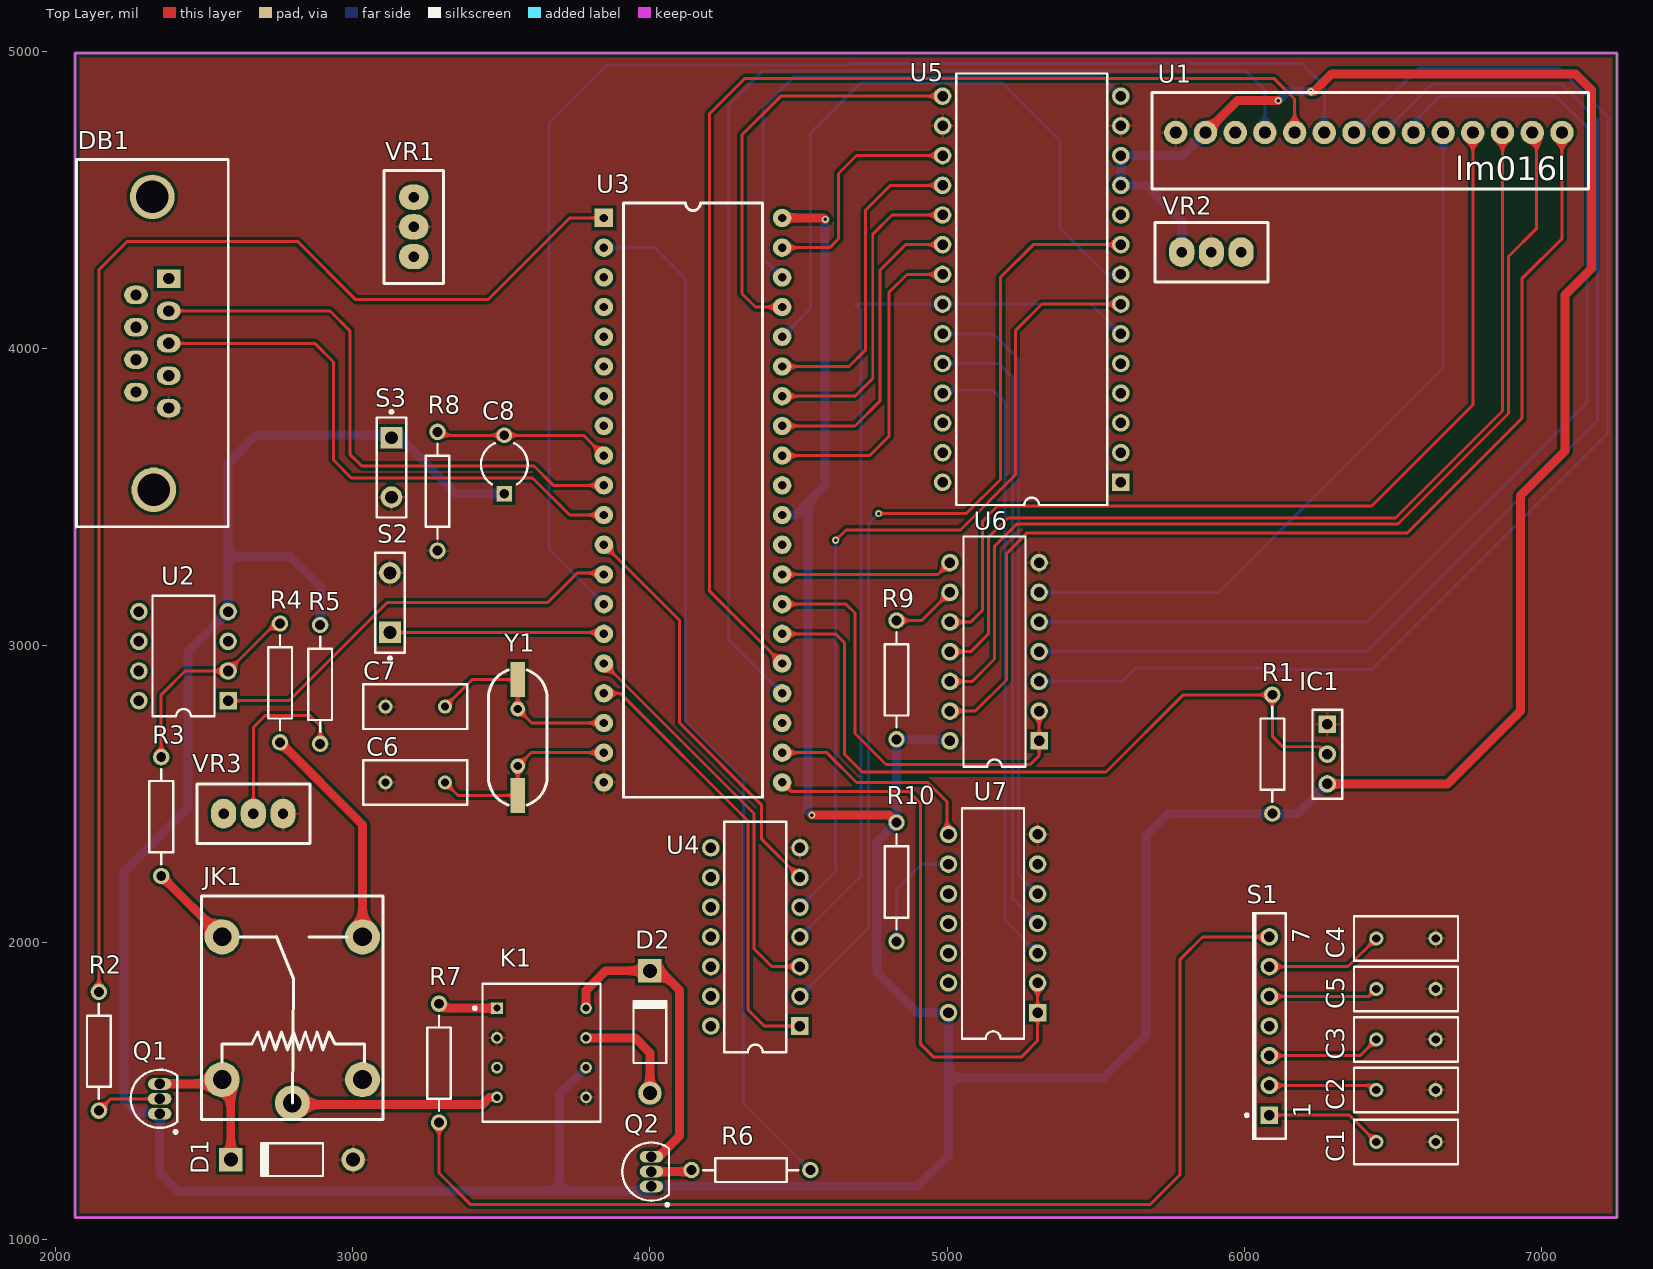
[diagram p0: Top Layer view]
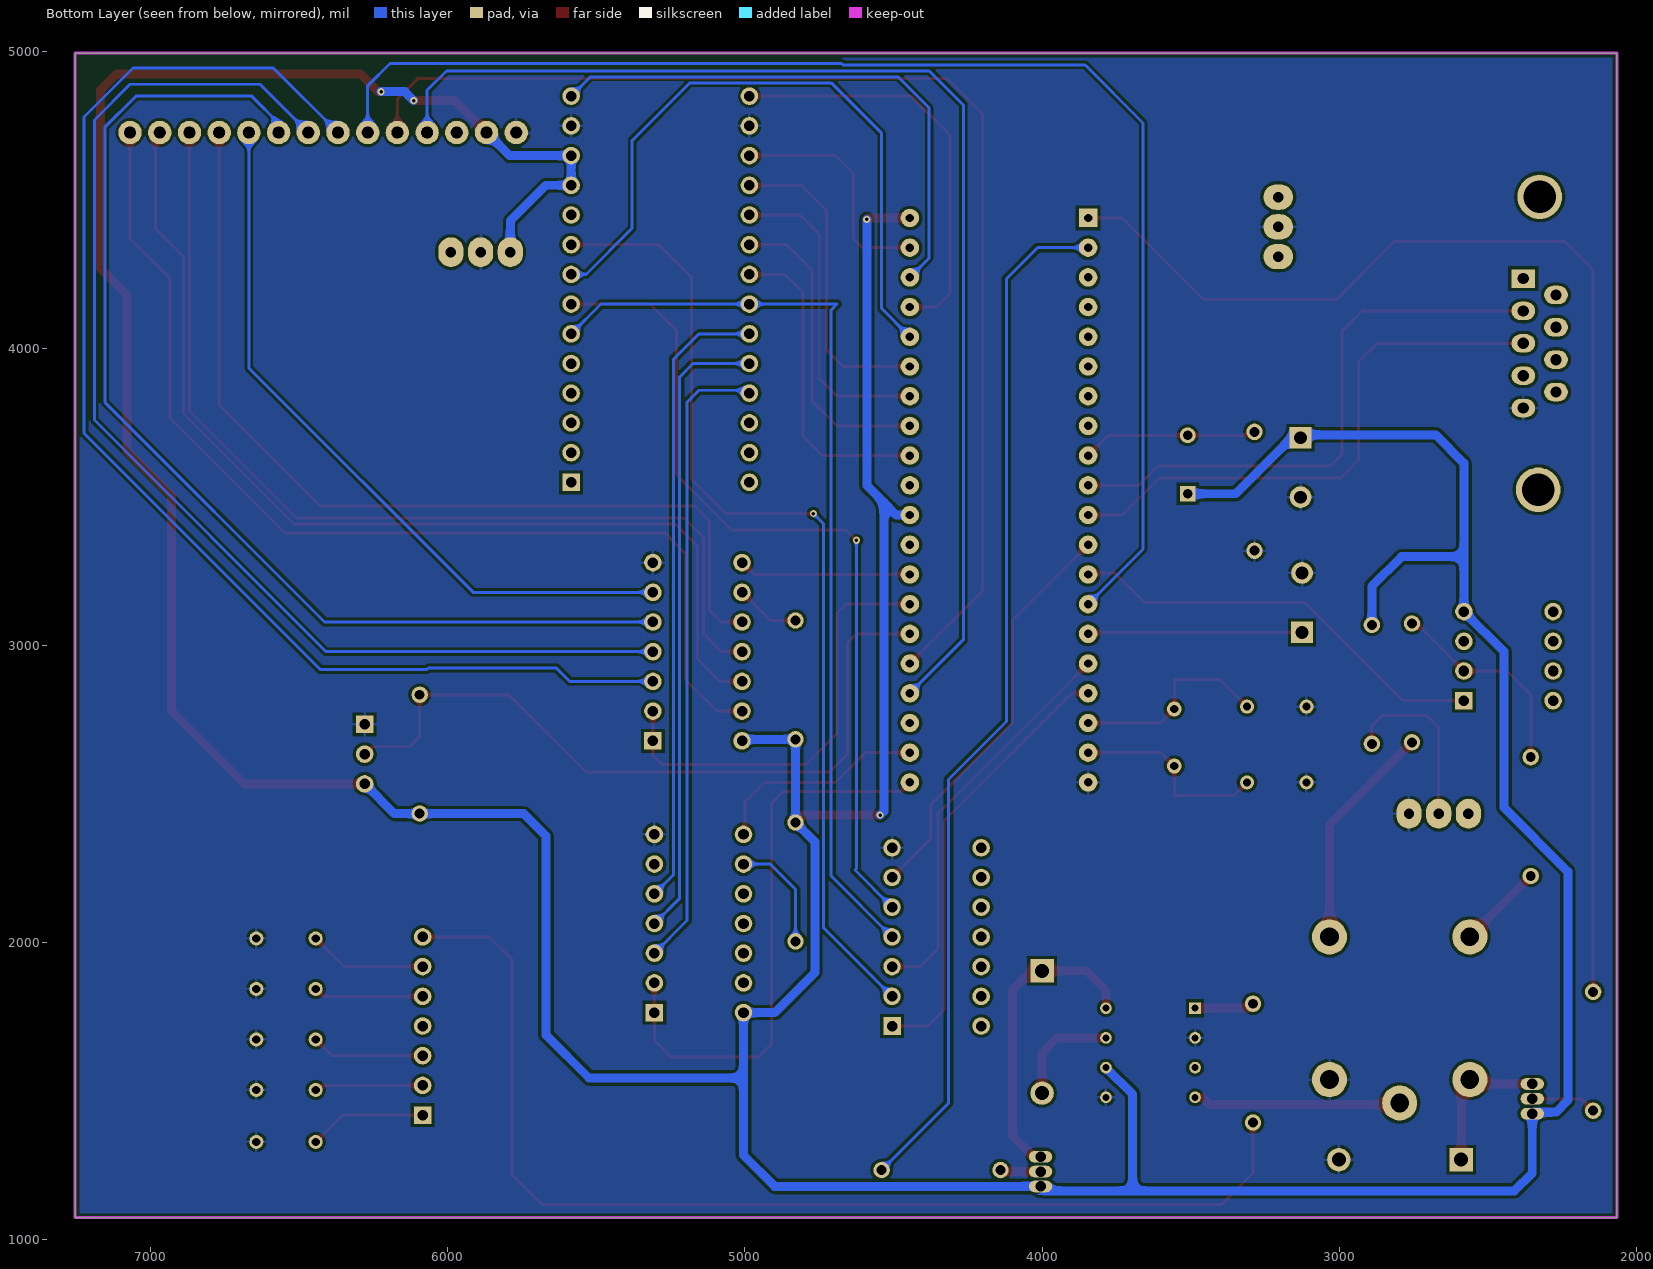
[diagram p1: Bottom Layer view, seen from below]
# Altium PCB MISC84284.PcbDoc
Units mil, origin at the board's own origin, x right, y up, seen from the top; angles counter-clockwise.
Board outline 5190 x 3920 mil, 2 copper layers (Top Layer, Bottom Layer); 40 components, 75 nets, 229 pads, 6 vias.

## Layer stack, top to bottom (the 12.6 mil dielectric is the usual default, probably not edited)
Top Solder: solder mask 0.4, Solder Resist, Dk 3.5
Top Layer: signal copper 1.4
Dielectric 1: dielectric 12.6, FR-4, Dk 4.8
Bottom Layer: signal copper 1.4
Bottom Solder: solder mask 0.4, Solder Resist, Dk 3.5

## Board outline
2065,1075 7255,1075 7255,4995 2065,4995

## Design rules (kind name [scope] priority, off if disabled: settings)
Clearance [All] p1: gap=10
MinimumSolderMaskSliver [All] p1: minsoldermaskwidth=0
PolygonConnect [All] p1: connectstyle=Relief reliefconductorwidth=10 reliefentries=4 polygonreliefangle="90 Angle" airgapwidth=10
RoutingVias [All] p1: holewidth=28 width=50 viastyle="Through Hole" minholewidth=28 minwidth=50 maxholewidth=28 maxwidth=50
SilkToSilkClearance [All] p1: silktosilkclearance=0
SilkToSolderMaskClearance [IsPad] p1: minsilkscreentomaskgap=0 clearancetoexposedcopper=TRUE
SolderMaskExpansion [All] p1: expansion=4
Width [All] p1: maxlimit=30 minlimit=10 preferedwidth=10
27 further rules are at their usual default settings.

## Classes and differential pairs
component class Sheet2: C6 C7 C8 DB1 R8 R9 R10 S3 U3 U4 U5 U6 U7 Y1
component class Sheet1: C1 C2 C3 C4 C5 D1 D2 IC1 JK1 K1 Q1 Q2 R1 R2 R3 R4 R5 R6 R7 S1 S2 U1 U2 VR1 VR2 VR3

## Components (designator, comment, footprint, x,y, rotation, side; value= is the part's Value field where it differs from the comment)
C1 "20NF" RAD-0.2 6545,1330 r180 top
C2 "200NF" RAD-0.2 6545,1505 r180 top
C3 "700NF" RAD-0.2 6545,1675 r180 top
C4 "67UF" RAD-0.2 6545,2015 r180 top
C5 "342UF" RAD-0.2 6545,1845 r180 top
C6 "30PF" RAD-0.2 3210,2540 r0 top
C7 "30PF" RAD-0.2 3210,2795 r0 top
C8 "10UF" CAPR5-4X5 3510,3610 r90 top
D1 "Diode 1N4001" DO-41 2795,1270 r180 top
D2 "Diode 1N4001" DO-41 4000,1700 r90 top
DB1 "DB9/F" DB9/F/180 2380,4236 r90 top
IC1 "DS18B20" HDR1X3 6280,2735 r270 top
JK1 "W172DIP-1" SRD-C_BK 2560,1539.68 r90 top
K1 "G2R-24-DC5" DIP-P8 3635,1630 r270 top
Q1 "2N3906" TO-92A 2350,1475 r0 top
Q2 "2N3906" TO-92A 4005,1230 r0 top
R1 "4.7K" AXIAL-0.4 6095,2635 r270 top
R2 "100" AXIAL-0.4 2145,1635 r90 top
R3 "10M" AXIAL-0.4 2355,2425 r270 top
R4 "10K" AXIAL-0.4 2755,2875 r270 top
R5 "1K" AXIAL-0.4 2890,2870 r270 top
R6 "100" AXIAL-0.4 4340,1235 r0 top
R7 "100" AXIAL-0.4 3290,1595 r90 top
R8 "10K" AXIAL-0.4 3285,3520 r90 top
R9 "10K" AXIAL-0.4 4830,2885 r270 top
R10 "10K" AXIAL-0.4 4830,2205 r90 top
S1 "SW-6WAY" SW-7 6085,1720 r90 top
S2 "SW-PB" SPST-2 3125,3145 r90 top
S3 "SW-PB" SPST-2 3130,3600 r270 top
U1 "LM016L" LM016L 6425,4700 r0 top
U2 "MAX942MJA" JA8 2430,2965 r90 top
U3 "AT89C51" DIP40 3845,4440 r0 top
U4 "SN74LS04N" 646-06 4355,2020 r90 top
U5 "ADC0808N" N028 5285,4200 r90 top
U6 "SN74LS164N" 646-06 5160,2980 r90 top
U7 "SN74LS164N" 646-06 5155,2065 r90 top
VR1 "RESVR" 3296W 3205,4410 r90 top
VR2 "RESVR" 3296W 5890,4325 r0 top
VR3 "4.7K" 3296W 2665,2435 r180 top
Y1 "12M" XTAL_US 3555,2787.13 r270 top

## Footprints (in the part's own frame and the unit in brackets; to place one, negate y for a bottom-side part, rotate by r counter-clockwise, add the part's x,y. Pads: shape width x height; smd on the part's side, far side on the other; paste and mask are expansions set on the pad)
646-06 [mm] "DIP; 14 Leads; Row Spacing 7.62 mm; Pitch 2.54 mm"
  rect 1.5x1.5 hole 0.9: 1(-7.62,-3.81)
  round 1.5 hole 0.9: 2(-5.08,-3.81) 3(-2.54,-3.81) 4(0,-3.81) 5(2.54,-3.81) 6(5.08,-3.81) 7(7.62,-3.81) 8(7.62,3.81) 9(5.08,3.81) 10(2.54,3.81) 11(0,3.81) 12(-2.54,3.81) 13(-5.08,3.81) 14(-7.62,3.81)
  silkscreen extent -9.85,-2.65 9.85,2.65
3296W [mil]
  oval 85x100 hole 35: 1(-100,0) 2(0,0) 3(100,0)
  silkscreen extent -190,-100 190,100, body extent -188,-94 188,94, height 455
AXIAL-0.4 [mm] "Axial Device, Thru-Hole; 2 Leads; 0.4 in Pin Spacing"
  round 1.4 hole 0.85: 1(-5.08,0) 2(5.08,0)
  silkscreen extent -4.06,-1.02 4.06,1.02
CAPR5-4X5 [mm] "Capacitor; 2 Leads"
  rect 1.35x1.35 hole 0.8: 1(-2.5,0)
  round 1.35 hole 0.8: 2(2.5,0)
  silkscreen extent -1.69,-2 1.82,2
DB9/F/180 [mil]
  round 150 hole 110: 0(-711,50) 0(275,55)
  rect 62x80 hole 38: 1(0,0)
  oval 62x80 hole 38: 2(-109,0) 3(-218,0) 4(-327,0) 5(-436,0) 6(-55,110) 7(-164,110) 8(-273,110) 9(-382,110)
  silkscreen extent -836,-200 400,310, body extent -830,-195 383,299, height 517
DIP40 [mil]
  rect 62x62 hole 28: 1(0,0)
  round 62 hole 28: 2(0,-100) 3(0,-200) 4(0,-300) 5(0,-400) 6(0,-500) 7(0,-600) 8(0,-700) 9(0,-800) 10(0,-900) 11(0,-1000) 12(0,-1100) 13(0,-1200) 14(0,-1300) 15(0,-1400) 16(0,-1500) 17(0,-1600) 18(0,-1700) 19(0,-1800) 20(0,-1900) 21(600,-1900) 22(600,-1800) 23(600,-1700) 24(600,-1600) 25(600,-1500) 26(600,-1400) 27(600,-1300) 28(600,-1200) 29(600,-1100) 30(600,-1000) 31(600,-900) 32(600,-800) 33(600,-700) 34(600,-600) 35(600,-500) 36(600,-400) 37(600,-300) 38(600,-200) 39(600,-100) 40(600,0)
  silkscreen extent 66,-1950 534,50
DIP-P8 [mm] "Dual-Pole Dual-Throw Relay; 8 Leads"
  rect 1x1 hole 0.6: 1(-3.81,-3.81)
  round 1 hole 0.6: 2(-1.27,-3.81) 3(1.27,-3.81) 4(3.81,-3.81) 5(3.81,3.81) 6(1.27,3.81) 7(-1.27,3.81) 8(-3.81,3.81)
  silkscreen extent -5.9,-5.82 5.9,5.05
DO-41 [mm] "Diode, Axial; Body 5.2 x 2.7 mm (LxDia. max), Lead Dia. 0.86 mm (max)"
  round 2 hole 1.2: 1(-5.23,0)
  rect 2x2 hole 1.2: 2(5.23,0)
  silkscreen extent -2.65,-1.4 2.75,1.4
HDR1X3 [mm] "Connector; Header; 3 Position"
  rect 1.5x1.5 hole 0.9: 1(0,0)
  round 1.5 hole 0.9: 2(2.54,0) 3(5.08,0)
  silkscreen extent -1.27,-1.27 6.35,1.27
JA8 [mm] "DIP; 8 Leads; Row Spacing 7.62 mm; Pitch 2.54 mm"
  rect 1.5x1.5 hole 0.9: 1(-3.81,-3.81)
  round 1.5 hole 0.9: 2(-1.27,-3.81) 3(1.27,-3.81) 4(3.81,-3.81) 5(3.81,3.81) 6(1.27,3.81) 7(-1.27,3.81) 8(-3.81,3.81)
  silkscreen extent -5.15,-2.65 5.15,2.65
LM016L [mm]
  round 2 hole 1 slot 1.005 at 0 deg paste+0 mask+0.051: 1(-16.637,0.699) 2(-14.097,0.699) 3(-11.557,0.699) 4(-9.017,0.699) 5(-6.477,0.699) 6(-3.937,0.699) 7(-1.397,0.699) 8(1.143,0.699) 9(3.683,0.699) 10(6.223,0.699) 11(8.763,0.699) 12(11.303,0.699) 13(13.843,0.699) 14(16.383,0.699)
  silkscreen extent -18.67,-4.13 18.67,4.13
N028 [mm] "DIP; 28 Leads; Row Spacing 15.24 mm; Pitch 2.54 mm"
  rect 1.5x1.5 hole 0.9: 1(-16.51,-7.62)
  round 1.5 hole 0.9: 2(-13.97,-7.62) 3(-11.43,-7.62) 4(-8.89,-7.62) 5(-6.35,-7.62) 6(-3.81,-7.62) 7(-1.27,-7.62) 8(1.27,-7.62) 9(3.81,-7.62) 10(6.35,-7.62) 11(8.89,-7.62) 12(11.43,-7.62) 13(13.97,-7.62) 14(16.51,-7.62) 15(16.51,7.62) 16(13.97,7.62) 17(11.43,7.62) 18(8.89,7.62) 19(6.35,7.62) 20(3.81,7.62) 21(1.27,7.62) 22(-1.27,7.62) 23(-3.81,7.62) 24(-6.35,7.62) 25(-8.89,7.62) 26(-11.43,7.62) 27(-13.97,7.62) 28(-16.51,7.62)
  silkscreen extent -18.45,-6.45 18.45,6.45
RAD-0.2 [mm] "Radial Cap, Thru-Hole; 2 Leads; 0.2 in Pin Spacing"
  round 1.2 hole 0.7: 1(-2.54,0) 2(2.54,0)
  silkscreen extent -4.44,-1.91 4.44,1.91
SPST-2 [mm] "Switch; 2 Leads"
  rect 1.85x1.85 hole 1.1: 1(-2.54,0)
  round 1.85 hole 1.1: 2(2.54,0)
  silkscreen extent -4.89,-1.27 4.28,1.27
SRD-C_BK [mm] "单刀双投"
  round 3 hole 1.6: 1(0,0) 2(0,-12) 3(-2,-6) 4(12.2,0) 5(12.2,-12)
  silkscreen extent -3.4,-13.75 15.7,1.75, body extent -3.4,-13.75 15.7,1.75, height 15.6
SW-7 [mm] "Switch; 7 Leads"
  rect 1.5x1.5 hole 0.9: 1(-7.62,0)
  round 1.5 hole 0.9: 2(-5.08,0) 3(-2.54,0) 4(0,0) 5(2.54,0) 6(5.08,0) 7(7.62,0)
  silkscreen extent -9.75,-1.4 9.75,2.05
TO-92A [mm] "TO, Flat Index; 3 In-Line, Axial Leads; Body Dia. 4.5mm; Leads 0.51 x 0.48 mm (max)"
  oval 2x1 hole 0.9: 1(0,-1.27) 2(0,0) 3(0,1.27)
  silkscreen extent -2.48,-2.95 1.5,2.48, body extent -2.48,-2.5 1.5,2.5, height 6.86
XTAL_US [mm]
  rect 3x1.27 smd: 1(-2.51,0) 2(7.39,0)
  round 1.27 hole 0.711: 1(0,0) 2(4.88,0)
  silkscreen extent -3.33,-2.5 8.21,2.5

## Part data
C1 C2 C3 C4 C5 C6 C7: library part Cap, "Capacitor"
C8: library part Cap2, "Capacitor"
D1 D2: "1 Amp General Purpose Rectifier"
IC1: "Digital thermometer"
JK1: library part SRD-S-105D, "5V一组转换"
K1: library part Relay-DPDT, "Dual-Pole Dual-Throw Relay"
Q1 Q2: "PNP General Purpose Amplifier"
R1 R2 R3 R4 R5 R6 R7 R8 R9 R10: library part Res2, "Resistor"
S1: "6 Way Switch"
S2 S3: "Switch"
U2: "High-speed, Low-power, 3V/5V, Rail-to-Rail Dual-Supply Comparator"
U3: "51 series MCU"
U4: "Hex Inverter"
U5: "CMOS Analog-to-Digital Converter with 8-Channel Multiplexer"
U6 U7: "Serial-In Parallel-Out Shift Register"
VR3: library part RESVR
Y1: library part XTAL, "Crystal Oscillator"

## Via types
v1: diameter 24, hole 12, Top Layer to Bottom Layer, 6 vias

## Nets (pads, with @x,y where several pads share a name; then routed paths per layer and width w, separated by ;. In a path a pad name is that pad's centre, name@x,y a point inside that pad or via, vN(x,y) a via of type N, cw(c..) or ccw(c..) an arc to the next point about the centre after c; other vN are vias at no path point)
+5V: VR1.1
A8: U5.25 U7.3 | length 2131.3
  Bottom Layer w10: U5.25 4995,3860 5155,3860 5195,3820 5195,2075 U7.3
A9: U5.24 U7.4 | length 2128.8
  Bottom Layer w10: U5.24 5175,3950 5220,3905 5220,2150 U7.4
A10: U5.23 U7.5 | length 2117.1
  Bottom Layer w10: U5.23 5155,4050 5240,3965 5240,2230 U7.5
AB1_LCD: U3.27 U6.1 U6.2 | length 1488.3
  Top Layer w10: U3.27 4660,3140 4690,3110 4690,2705 4795,2600 5280,2600 5310,2630 U6.1 U6.2
AB2_ADC: U3.21 U7.1 U7.2 | length 1935.4
  Top Layer w10: U3.21 4475,2510 4870,2510 4910,2470 4910,1660 4955,1615 5250,1615 5305,1670 U7.1 U7.2
CAPC1: C1.2 S1.1 | length 397.3
  Top Layer w10: S1.1 6355,1420 C1.2
CAPC2: C2.2 S1.2 | length 366.2
  Top Layer w10: S1.2 6430,1520 C2.2
CAPC3: C3.2 S1.3 | length 382.8
  Top Layer w10: S1.3 6390,1620 C3.2
CAPC4: C4.2 S1.6 | length 399.4
  Top Layer w10: S1.6 6350,1920 C4.2
CAPC5: C5.2 S1.5 | length 370.4
  Top Layer w10: S1.5 6420,1820 C5.2
CC: R7.1 S1.7 | length 3806
  Top Layer w10: R7.1 3290,1225 3395,1120 5685,1120 5785,1220 5785,1945 5860,2020 S1.7
CLK1_LCD: U3.28 U6.8 | length 581.6
  Top Layer w10: U3.28 4970,3240 U6.8
CLK2_ADC: U3.22 U7.8 | length 735.4
  Top Layer w10: U3.22 4595,2640 4695,2540 4935,2540 5000,2475 5000,2370 U7.8
COM: JK1.3 K1.4 | length 704.2
  Top Layer w30: JK1.3 2796.22,1455.63 3435.63,1455.63 3460,1480 K1.4
D0: U1.7 U6.3 | length 4343.4
  Bottom Layer w10: U6.3 5590,2880 5635,2925 6065,2925 6070,2920 6430,2920 7225,3715 7225,4780 7060,4945 6587.5,4945 U1.7
D1: U1.8 U6.4 | length 4050.1
  Bottom Layer w10: U6.4 6410,2980 7190,3760 7190,4770 7070,4890 6632.5,4890 U1.8
D2: U1.9 U6.5 | length 3774.8
  Bottom Layer w10: U6.5 6415,3080 7155,3820 7155,4745 7050,4850 6660,4850 6570,4760 U1.9
D3: U1.10 U6.6 | length 2465.2
  Bottom Layer w10: U6.6 5915,3180 6670,3935 U1.10
D4: U1.11 U6.10 | length 3155.6
  Top Layer w10: U6.10 5080,3080 5120,3120 5120,3420 5170,3470 6430,3470 6770,3810 U1.11
D5: U1.12 U6.11 | length 3323.4
  Top Layer w10: U6.11 5080,2980 5140,3040 5140,3365 5205,3430 6510,3430 6870,3790 U1.12
D6: U1.13 U6.12 | length 3467.4
  Top Layer w10: U6.12 5085,2880 5160,2955 5160,3335 5235,3410 6518.28,3410 6890,3781.72 6890,4310 6985,4405 6985,4712.5 U1.13
D7: U1.14 U6.13 | length 3600.4
  Top Layer w10: U6.13 5095,2780 5200,2885 5200,3310 5270,3380 6550,3380 6935,3765 6935,4235 7070,4370 U1.14
DAT0: U3.39 U5.17 | length 797.3
  Top Layer w10: U3.39 4605,4340 4635,4370 4635,4590 4695,4650 U5.17
DAT1: U3.38 U5.14 | length 1872.3
  Bottom Layer w10: U3.38 4380,4305 4380,4810 4485,4915 5520,4915 U5.14
DAT2: U3.37 U5.15 | length 1417.5
  Top Layer w10: U3.37 4355,4140 4310,4185 4310,4720 4440,4850 U5.15
DAT3: U3.36 U5.8 | length 2279.7
  Bottom Layer w10: U3.36 4540,4135 4540,4725 4710,4895 5185,4895 5380,4700 5380,4405 5535,4250 U5.8
DAT4: U3.35 U5.18 | length 1068
  Top Layer w10: U3.35 4670,3940 4725,3995 4725,4465 4810,4550 U5.18
DAT5: U3.34 U5.19 | length 1076.8
  Top Layer w10: U3.34 4690,3840 4750,3900 4750,4385 4815,4450 U5.19
DAT6: U3.33 U5.20 | length 1050.4
  Top Layer w10: U3.33 4690,3740 4775,3825 4775,4265 4860,4350 U5.20
DAT7: U3.32 U5.21 | length 1076.8
  Top Layer w10: U3.32 4740,3640 4805,3705 4805,4190 4865,4250 U5.21
E: U1.6 U3.14 | length 4578
  Bottom Layer w10: U3.14 3660,3325 3660,4760 3855,4955 4670,4955 4675,4960 6195,4960 6270,4885 U1.6
EOC: U4.5 U5.7 | length 2862.3
  Top Layer w10: v1(4625,3355) 4660,3390 5045,3390 5230,3575 5230,4060 5320,4150 U5.7
  Bottom Layer w10: U4.5 4630,2245 4625,2250 v1(4625,3355)
GND: C1.1 C2.1 C3.1 C4.1 C5.1 C6.1 C7.1 D1.1 DB1.5 IC1.1 JK1.2 K1.2 K1.5 R8.1 S2.2 S3.2 U1.1 U3.20 U4.7 U5.13 U5.16 U6.7 U7.7 VR1.2 VR2.2 VR3.1
IN0: U5.26
INT0: U3.12 U4.6 | length 1393.4
  Top Layer w10: U3.12 4100,3085 4100,2740 4375,2465 4375,2350 U4.6
KEY: S2.1 U3.15 | length 722.1
  Top Layer w10: S2.1 3840,3045 U3.15
NetC6_2: C6.2 U3.19 Y1.2 | length 670.6
  Top Layer w10: C6.2 3353.82,2496.18 3555,2496.18 3555,2595 3600,2640 U3.19
NetC7_2: C7.2 U3.18 Y1.1 | length 691
  Top Layer w10: C7.2 3400.94,2885.94 3555,2885.94 3555,2787.13 3602.13,2740 U3.18
NetC8_2: C8.2 R8.2 U3.9 | length 593.1
  Top Layer w10: R8.2 3296.57,3708.43 C8.2 3776.57,3708.43 U3.9
NetD1_2: D1.2 JK1.1 Q1.3 | length 497.8
  Top Layer w30: Q1.3 2545.32,1525 JK1.1 2589.09,1510.59 D1.2
NetD2_1: D2.1 K1.7 | length 371.6
  Top Layer w30: K1.7 3950,1680 4000,1630 D2.1
NetD2_2: D2.2 K1.8 Q2.3 | length 1043.6
  Top Layer w30: K1.8 3785,1840 3850.91,1905.91 D2.2 4034.09,1905.91 4100,1840 4100,1350 4030,1280 Q2.3
NetK1_1: K1.1 R7.2 | length 201.2
  Top Layer w30: R7.2 3305,1780 K1.1
NetQ1_2: Q1.2 R2.1 | length 221.6
  Top Layer w10: R2.1 2185,1475 Q1.2
NetQ2_2: Q2.2 R6.1 | length 137.1
  Top Layer w30: Q2.2 4135,1230 R6.1
NetR3_1: R3.1 R4.1 U2.2 | length 709.4
  Top Layer w10: R3.1 2355,2835 2435,2915 U2.2 2740,3075 R4.1
NetR5_2: R5.2 VR3.2 | length 606.1
  Top Layer w10: VR3.2 2665,2725 2705,2765 2855,2765 2890,2730 R5.2
NetR9_1: R9.1 U6.9 | length 219.4
  Top Layer w10: R9.1 4915,3085 U6.9
NetR10_1: R10.1 U7.9 | length 385.2
  Bottom Layer w10: R10.1 4830,2180 4915,2265 U7.9
NetU1_3: U1.3
NetU2_3: U2.3
NF: JK1.4 R3.2 | length 289.9
  Top Layer w30: R3.2 JK1.4
OE: U4.2 U5.9 | length 3323
  Top Layer w10: v1(4770,3445) 5065,3445 5180,3560 5180,4240 5290,4350 U5.9
  Bottom Layer w10: U4.2 4735,2050 4735,3410 v1(4770,3445)
P10: R2.2 U3.1 | length 4364
  Top Layer w10: R2.2 2145,4265 2240,4360 2815,4360 3010,4165 3455,4165 3730,4440 U3.1
P11: R6.2 U3.2 | length 3492.5
  Bottom Layer w10: U3.2 4015,4340 4120,4235 4120,2745 4315,2550 4315,1460 R6.2
P12: U3.3
P13: U3.4
P14: U3.5
P15: U3.6
P16: U3.7
P17: U3.8
P25: IC1.2 R1.1 U3.26 | length 2519.8
  Top Layer w10: U3.26 4625,3040 4655,3010 4655,2635 4715,2575 5535,2575 5795,2835 R1.1 6095,2695 6130,2660 6255,2660 IC1.2
P33: U2.1 U3.13 | length 1445.2
  Top Layer w10: U2.1 2785,2815 3115,3145 3655,3145 3755,3245 3840,3245 U3.13
RD: U3.17 U4.1 | length 1495.9
  Top Layer w10: U3.17 3900,2840 4330,2410 4330,1775 4385,1720 U4.1
RS: U1.4 U3.24 | length 4076.6
  Bottom Layer w10: U3.24 4265,3020 4265,4820 4380,4935 6005,4935 6070,4870 U1.4
RW: U1.5 U3.25 | length 4112.7
  Top Layer w10: U3.25 4200,3185 4200,4790 4320,4910 6100,4910 6170,4840 U1.5
RXD: DB1.2 U3.10 | length 1951.2
  Top Layer w10: DB1.2 2923,4127 2990,4060 2990,3645 3030,3605 3610,3605 3675,3540 U3.10
START: U4.4 U5.6 U5.22 | length 3159.6
  Bottom Layer w10: U4.4 4710,2225 4710,4130 4690,4150 U5.22 5485,4150 U5.6
TXD: DB1.3 U3.11 | length 1897.7
  Top Layer w10: DB1.3 2872,4018 2935,3955 2935,3625 2995,3565 3605,3565 3730,3440 U3.11
UF: JK1.5 R4.2 | length 769.9
  Top Layer w30: R4.2 3032.44,2397.56 JK1.5
VCC: C8.1 IC1.3 K1.6 Q1.1 Q2.1 R1.2 R5.1 R9.2 R10.2 S3.1 U1.2 U2.4 U3.30 U3.40 U5.11 U5.12 U6.14 U7.14 VR2.1 | length 18894.7
  Top Layer w30: U3.40 4585,4440 v1(4590,4435) ; v1(4545,2430) 4805,2430 R10.2 ; U1.2 5977.5,4835 v1(6115,4835) ; v1(6225,4865) 6235,4865 6295,4925 7115,4925 7170,4870 7170,4270 7080,4180 7080,3655 6930,3505 6930,2780 6685,2535 IC1.3
  Bottom Layer w30: R5.1 2890,3200 2790,3300 2580,3300 ; C8.1 3348.43,3511.57 3160,3700 S3.1 3120,3710 2675,3710 2580,3615 2580,3300 ; K1.6 3695,1490 3695,1165 ; U3.30 4490,3440 4532.5,3482.5 ; v1(4545,2430) 4532.5,2442.5 4532.5,3482.5 ; v1(4590,4435) 4590,3540 4532.5,3482.5 ; U6.14 5005,2685 R9.2 R10.2 4765,2340 4765,1900 4900,1765 U7.14 5005,1545 ; VR2.1 5790,4430 5670,4550 U5.11 U5.12 5792.5,4650 U1.2 ; v1(6115,4835) 6145,4865 v1(6225,4865) ; IC1.3 6180,2435 R1.2 5745,2435 5670,2360 5670,1690 5525,1545 5005,1545 ; 2580,3300 U2.4 2445,2980 2445,2455 2230,2240 2230,1470 2270,1430 2345,1430 Q1.1 2350,1225 2410,1165 3695,1165 ; 3695,1165 3990,1165 Q2.1 4900,1180 5005,1285 5005,1545
VDD: U4.14
VEE: U2.8
WR: U3.16 U4.3 | length 1349
  Top Layer w10: U3.16 4350,2435 4350,1980 4410,1920 U4.3
pads on no net: DB1.0 DB1.1 DB1.4 DB1.6 DB1.7 DB1.8 DB1.9 K1.3 S1.4 U2.5 U2.6 U2.7 U3.23 U3.29 U3.31 U4.8 U4.9 U4.10 U4.11 U4.12 U4.13 U5.1 U5.2 U5.3 U5.4 U5.5 U5.10 U5.27 U5.28 U7.6 U7.10 U7.11 U7.12 U7.13 VR1.3 VR2.3 VR3.3

## Polygon pours and split planes (outlines as drawn)
GND on Top Layer "D" (solid, remove dead copper, pour order 0): 1465,5290 1565,5390 8065,5390 8065,1550 7325,810 7105,1030 1130,1030
GND on Bottom Layer "D" (solid, remove dead copper, pour order 2): 1040,5240 7835,5240 7910,5315 7730,5135 7730,760 1220,760 1120,660

## Keep-outs
Keep-Out Layer:
  lines w10: 2065,1075 7000,1075 7255,1075 7255,4995 2065,4995 2065,4635 2065,1125 2065,1075